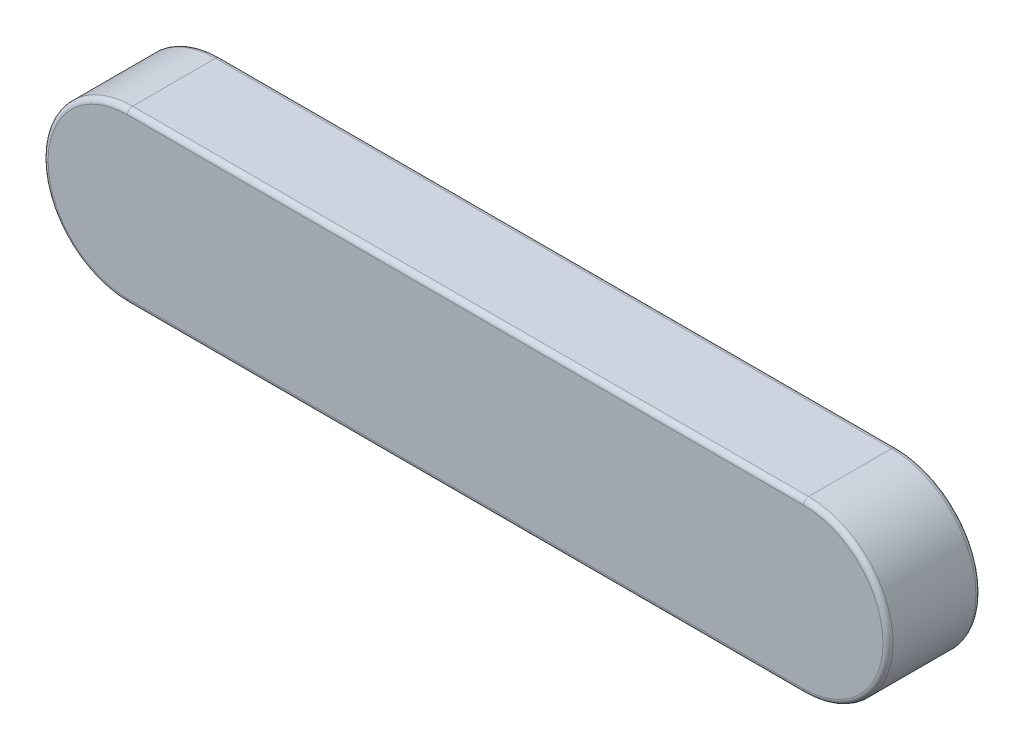
SolidWorks part; units mm, degrees
ref_plane "Plane1" through (0, 0, 0) normal (0, 0, 1) x (1, 0, 0)
ref_plane "Plane2" through (0, 0, 0) normal (0, 1, 0) x (1, 0, 0)
ref_plane "Plane3" through (0, 0, 0) normal (1, 0, 0) x (0, 0, -1)
sketch "Dimension Sketch" plane through (0, 0, 0) normal (0, 0, 1) x (1, 0, 0)
  line L0 (-100, 0) -> (100, 0) construction
  point P3 (-22, 0)
  point P4 (-1.2, 0)
  point P5 (0, 0)
  point P8 (-40, 0)
  point P11 (0, 0)
sketch "Sketch1" plane through (0, 0, 0) normal (0, 0, 1) x (1, 0, 0)
  line L0 (-28.0599, 0) -> (30.562, 0) construction
  line L1 (-80, 20) -> (80, 20)
  line L2 (-80, -20) -> (80, -20)
  line L3 (0, 2.9108) -> (0, -2.1805) construction
  arc A0 (-80, 20) -> (-80, -20) centre (-80, 0) ccw
  arc A1 (80, 20) -> (80, -20) centre (80, 0) cw
extrude "Base-Extrude" add sketch "Sketch1" along normal blind 22
fillet "Fillet1" radius 1.2 8 edges at (100, 0, 22) (0, 20, 22) (-100, 0, 22) (0, 20, 0) (100, 0, 0) (0, -20, 0) (-100, 0, 0) (0, -20, 22)
equation "\"D3@Sketch1\" = \"L@Dimension Sketch\""
equation "\"D1@Sketch1\" = \"b@Dimension Sketch\" / 2"
equation "\"D1@Fillet1\" = \"r@Dimension Sketch\""
equation "\"D1@Base-Extrude\" = \"h@Dimension Sketch\""
